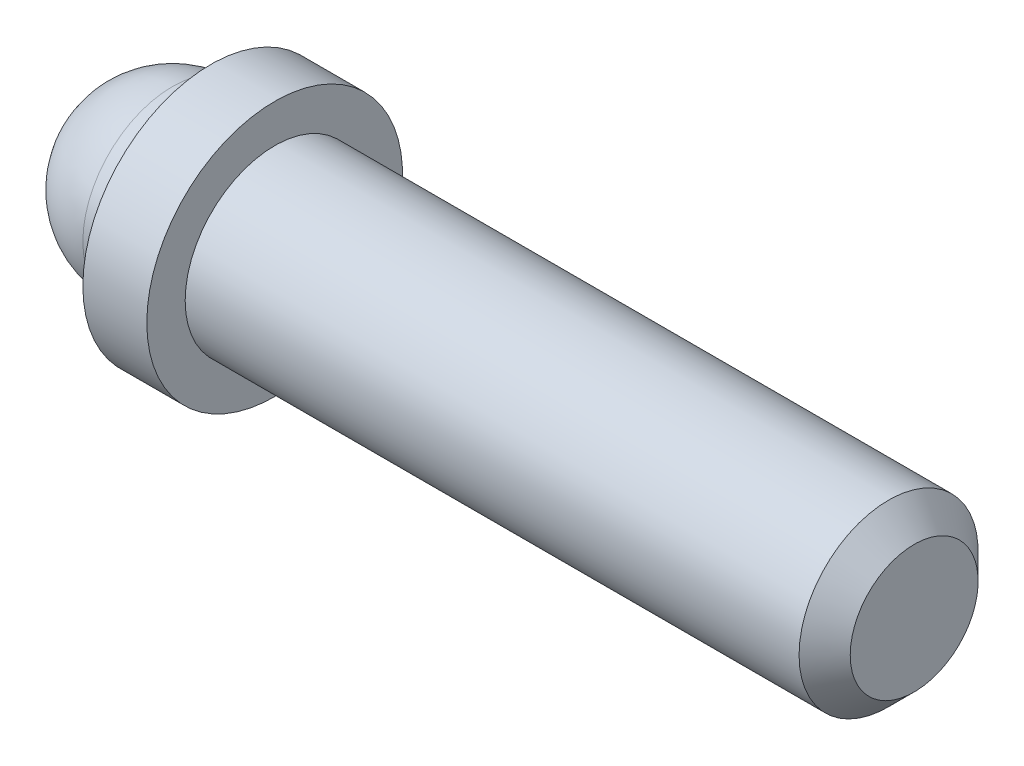
from build123d import *


with BuildPart() as part:
    # Sketch1 → Revolve1 (revolve)
    with BuildSketch(Plane.XY, mode=Mode.PRIVATE) as revolve1_sk:
        with BuildLine():
            Line((0, 0), (0, 5))
            Line((0, 5), (-2, 7))
            Line((-2, 7), (-50, 7))
            Line((-50, 7), (-50, 10))
            Line((-50, 10), (-55, 10))
            Line((-55, 10), (-55, 7))
            Line((-55, 7), (-58, 7))
            ThreePointArc((-58, 7), (-62.949747468, 4.949747468), (-65, 0))
            Line((-65, 0), (0, 0))
        make_face()
    revolve(revolve1_sk.sketch.rotate(Axis((-89.758555814, 0, 0), (1, 0, 0)), 90), axis=Axis((-89.758555814, 0, 0), (1, 0, 0)))


solid = part.part
